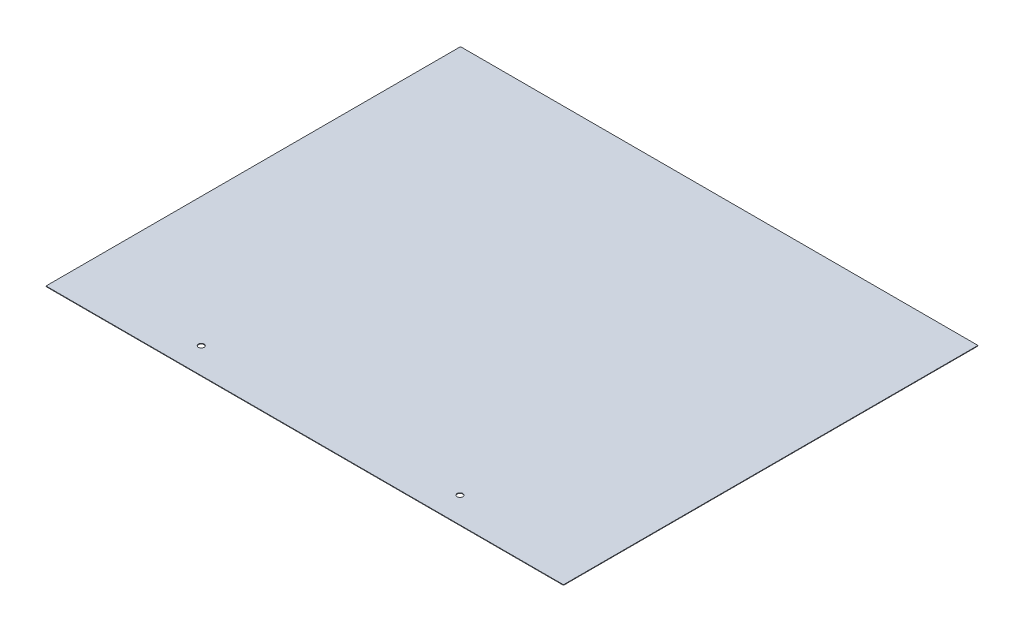
SolidWorks part; units mm, degrees
ref_plane "Front Plane" through (0, 0, 0) normal (0, 0, 1) x (1, 0, 0)
ref_plane "Top Plane" through (0, 0, 0) normal (0, 1, 0) x (1, 0, 0)
ref_plane "Right Plane" through (0, 0, 0) normal (1, 0, 0) x (0, 0, -1)
sketch "Sketch1" plane through (0, 0, 0) normal (0, 1, 0) x (1, 0, 0)
  line L1 (-500, -400.5) -> (500, -400.5)
  line L2 (-500, -400.5) -> (-500, 400.5)
  line L3 (-500, 400.5) -> (500, 400.5)
  line L4 (500, -400.5) -> (500, 400.5)
  line L5 (-500, -400.5) -> (500, 400.5) construction
  line L6 (-500, 400.5) -> (500, -400.5) construction
  point P0 (0, 0)
  dimension "D1" = 1000
  dimension "D2" = 801
extrude "Boss-Extrude1" add sketch "Sketch1" along normal blind 1
sketch "Sketch2" plane through (0, 1, 0) normal (0, 1, 0) x (1, 0, 0)
  line L1 (-500, -400.5) -> (500, -400.5) construction
  circle A0 centre (-250, -350.5) radius 5.5
  circle A1 centre (250, -350.5) radius 5.5
  dimension "D1" = 50
  dimension "D2" = 50
  dimension "D3" = 500
  dimension "D4" = 11
extrude "Cut-Extrude1" cut sketch "Sketch2" against normal through all
